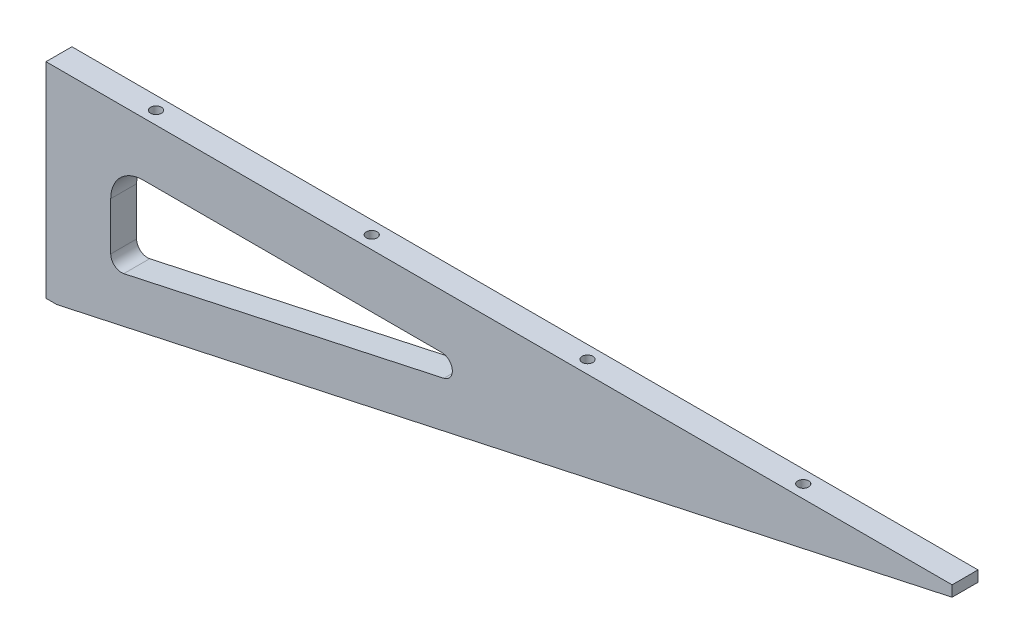
SolidWorks part; units mm, degrees
ref_plane "Front Plane" through (0, 0, 0) normal (0, 0, 1) x (1, 0, 0)
ref_plane "Top Plane" through (0, 0, 0) normal (0, 1, 0) x (1, 0, 0)
ref_plane "Right Plane" through (0, 0, 0) normal (1, 0, 0) x (0, 0, -1)
sketch "Sketch1" plane through (0, 0, 0) normal (0, 0, 1) x (1, 0, 0)
  line L0 (0, -95) -> (0, 0)
  line L1 (0, 0) -> (420, 0)
  line L2 (420, -5) -> (5, -95)
  line L3 (420, 0) -> (420, -5)
  line L4 (5, -95) -> (0, -95)
  line L5 (30, -62.1729) -> (30, -40)
  line L6 (45, -25) -> (183.3529, -25)
  line L7 (184.4127, -34.8864) -> (36.0597, -67.0593)
  arc A0 (45, -25) -> (30, -40) centre (45, -40) ccw
  arc A1 (30, -62.1729) -> (36.0597, -67.0593) centre (35, -62.1729) ccw
  arc A2 (183.3529, -25) -> (184.4127, -34.8864) centre (183.3529, -30) cw
  point P11 (30, -25)
  point P16 (230, -25)
  dimension "D8" = 15
  dimension "D9" = 5
  dimension "D1" = 5
  dimension "D2" = 5
  dimension "D3" = 95
  dimension "D4" = 420
  dimension "D5" = 200
  dimension "D6" = 30
  dimension "D7" = 25
extrude "Boss-Extrude1" add sketch "Sketch1" along normal blind 12
hole_wizard "M6 Tapped Hole1" positions "Sketch3" profile "Sketch2" tap size "M6" standard "Gb"
sketch "Sketch3" plane through (0, 0, 0) normal (-1, 0, 0) x (0, 0, 1)
  line L0 (12, -47.5) -> (-24.0233, -47.5) construction
  line L1 (12, 0) -> (12, -95) construction
  line L3 (6, 0) -> (6, -32.7081) construction
  line L4 (12, 0) -> (0, 0) construction
  point P0 (6, -15)
  point P2 (6, -47.5)
  point P4 (6, -80)
  dimension "D1" = 65
sketch "Sketch2" plane through (0, -15, 6) normal (0, 1, 0) x (0, 0, 1)
  line L0 (0, 0) -> (0, 16.5022)
  line L1 (0, 16.5022) -> (2.5, 15)
  line L2 (2.5, 15) -> (2.5, 0)
  line L5 (2.5, 0) -> (0, 0)
  line L10 (0, 16.5022) -> (-2.5, 15) construction
  line L11 (0, -6.35) -> (0, 107.95) construction
  dimension "螺纹孔钻头直径" = 5
  dimension "螺纹孔钻头深度" = 15
  dimension "导头角度" = 118
cosmetic thread "Cosmetic Thread1" parameters "D1"=12, "D2"=6
cosmetic thread "Cosmetic Thread2" parameters "D1"=12, "D2"=6
cosmetic thread "Cosmetic Thread3" parameters "D1"=12, "D2"=6
hole_wizard "M6 Tapped Hole2" positions "Sketch5" profile "Sketch4" tap size "M6" standard "Gb"
sketch "Sketch5" plane through (0, 0, 0) normal (0, 1, 0) x (-1, 0, 0)
  line L0 (0, 12) -> (0, 0) construction
  line L2 (0, 6) -> (-29.335, 6) construction
  point P0 (-45, 6)
  point P11 (-145, 6)
  point P12 (-245, 6)
  point P13 (-345, 6)
  dimension "D1" = 45
  dimension "D2" = 4
sketch "Sketch4" plane through (45, 0, 6) normal (1, 0, 0) x (0, 0, 1)
  line L0 (0, 0) -> (0, 16.5022)
  line L1 (0, 16.5022) -> (2.5, 15)
  line L2 (2.5, 15) -> (2.5, 0)
  line L5 (2.5, 0) -> (0, 0)
  line L10 (0, 16.5022) -> (-2.5, 15) construction
  line L11 (0, -6.35) -> (0, 107.95) construction
  dimension "螺纹孔钻头直径" = 5
  dimension "螺纹孔钻头深度" = 15
  dimension "导头角度" = 118
cosmetic thread "Cosmetic Thread4" parameters "D1"=12, "D2"=6
cosmetic thread "Cosmetic Thread5" parameters "D1"=12, "D2"=6
cosmetic thread "Cosmetic Thread6" parameters "D1"=12, "D2"=6
cosmetic thread "Cosmetic Thread7" parameters "D1"=12, "D2"=6
